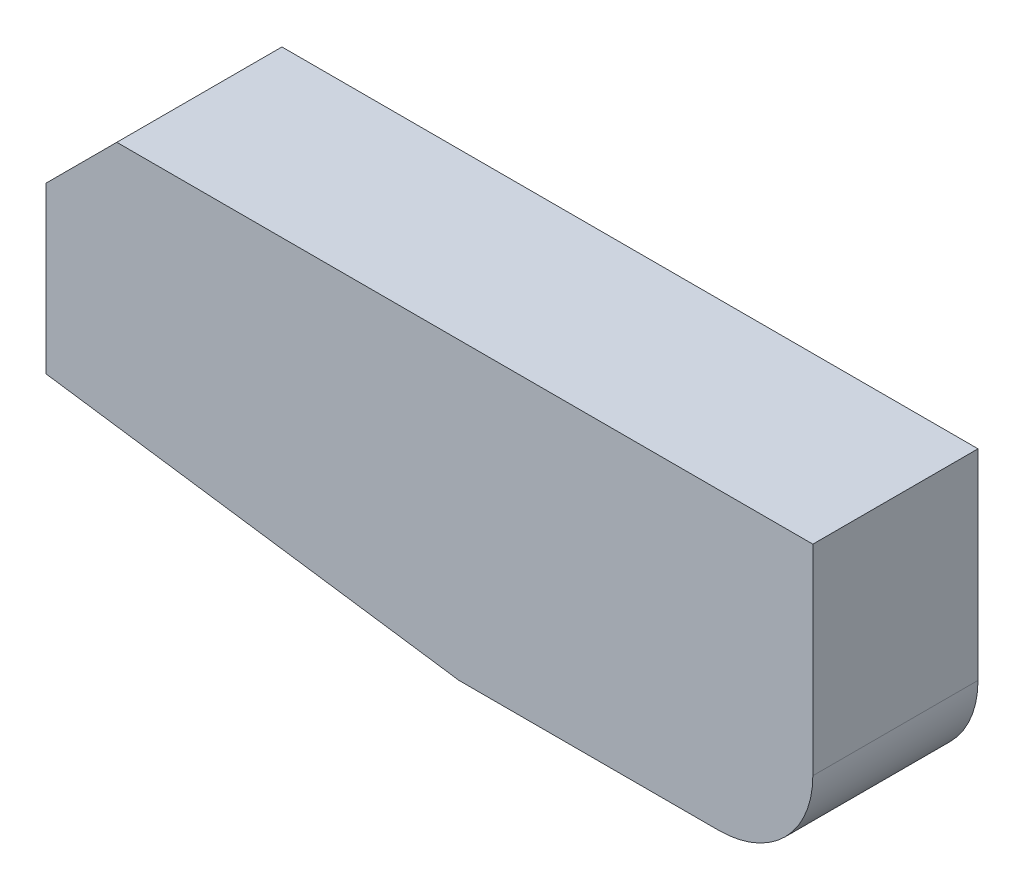
SolidWorks part; units mm, degrees
material "普通碳钢"
ref_plane "前视" through (0, 0, 0) normal (0, 0, 1) x (1, 0, 0)
ref_plane "上视" through (0, 0, 0) normal (0, 1, 0) x (1, 0, 0)
ref_plane "右视" through (0, 0, 0) normal (1, 0, 0) x (0, 0, -1)
sketch "草图1" plane through (0, 0, 0) normal (0, 0, 1) x (1, 0, 0)
  line L0 (-100.4567, 0) -> (65, 0) construction
  line L1 (0, 69.0325) -> (0, -66.5084) construction
  line L2 (0, 5) -> (0, 25)
  line L3 (0, 5) -> (35, 0)
  line L4 (0, 25) -> (65, 25)
  line L5 (65, 25) -> (65, 0)
  line L6 (35, 0) -> (65, 0)
  dimension "D1" = 65
  dimension "D2" = 35
  dimension "D3" = 20
  dimension "D4" = 25
extrude "凸台-拉伸1" add sketch "草图1" along normal mid plane 14
chamfer "倒角1" distance 6 angle 45 1 edges at (0, 25, 0)
fillet "圆角1" radius 8 1 edges at (65, 0, 0)
